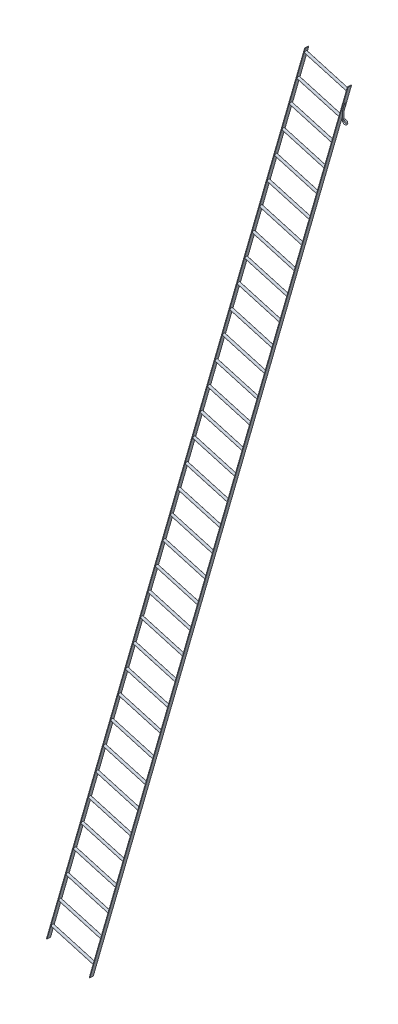
from build123d import *

# Parameters (mm, degrees)
SWEEP2_PROFILE_R                              = 6
CHAMFER1_SIZE                                 = 0.5
SKETCH1_W                                     = 40
SKETCH1_H                                     = 6
GB_T_704_1988HOT_ROLLED_FLAT_STEEL_40_6_DEPTH = 10400
SKETCH1_ON_SEGMENT_2_W                        = 40
SKETCH1_ON_SEGMENT_2_H                        = 6
GB_T_704_1988HOT_ROLLED_FLAT_STEEL_4_2_DEPTH  = 10400
SKETCH13_R                                    = 13.4
SKETCH13_R_2                                  = 10.4
GB_T_6728_2002ROUND_TUBE_26_8_X_3_2_DEPTH     = 494
SKETCH13_ON_SEGMENT_2_R                       = 13.4
SKETCH13_ON_SEGMENT_2_R_2                     = 10.4
GB_T_6728_2002ROUND_TUBE_26_8_X_3_2_2_DEPTH   = 494
PATTERN_LINEAR_1_COUNT                        = 34
PATTERN_LINEAR_1_PITCH                        = 300


with BuildPart() as part:
    # Sweep2: sweep along a path in feature 17 (ProfileFeature) (+16 more in 12 files) Sketch1
    with BuildLine(Plane.XY) as sweep2_path:
        Line((2.366140089, 179), (-19.767570176, 101.810579127))
        ThreePointArc((-19.767570176, 101.810579127), (-19.941608412, 100.991793598), (-20, 100.156754992))
        Line((-20, 100.156754992), (-20, 0))
        ThreePointArc((-20, 0), (14.142135624, -14.142135624), (0, 20))
        Line((0, 20), (-13.95, 20))
    # Sweep2 profile (on start of the path) → Sweep2 (sweep)
    with BuildSketch(Plane(origin=(2.366140089, 179, 0), x_dir=(-0.9612616959383187, 0.27563735581700005, 0), z_dir=(-0.27563735581700005, -0.9612616959383187, 0))):
        Circle(SWEEP2_PROFILE_R)
    sweep(path=sweep2_path.line)

    # Chamfer1
    chamfer1_edges = [part.edges().sort_by_distance(p)[0] for p in [
        (8.133710265, 177.346175865, 0),
    ]]
    chamfer(chamfer1_edges, length=CHAMFER1_SIZE)


with BuildPart() as body_2:
    # Sketch1 → Gb／t 704—1988Hot-rolled Flat Steel 40×6(1) (new body)
    with BuildSketch(Plane(origin=(-2816.280646199, -9629.021782916, -20), x_dir=(0, 0, 1), z_dir=(-0.27563735581699317, -0.9612616959383207, 0))):
        with Locations((20, 3)):
            Rectangle(SKETCH1_W, SKETCH1_H)
    extrude(amount=-GB_T_704_1988HOT_ROLLED_FLAT_STEEL_40_6_DEPTH)


with BuildPart() as body_3:
    # Sketch1 on segment 2 (carried to segment 2) → Gb_t 704_1988Hot-rolled Flat Steel 4 2 (new body)
    with BuildSketch(Plane(origin=(-424.515423496, 504.264708616, -20), x_dir=(0, 0, 1), z_dir=(-0.275637356, -0.961261696, 0))):
        with Locations((20, 3)):
            Rectangle(SKETCH1_ON_SEGMENT_2_W, SKETCH1_ON_SEGMENT_2_H)
    extrude(amount=GB_T_704_1988HOT_ROLLED_FLAT_STEEL_4_2_DEPTH)


with BuildPart() as body_4:
    # Sketch13 → Gb／t 6728—2002Round Tube 26.8 X 3(2) (new body)
    with BuildSketch(Plane(origin=(-3249.79832062, -9348.667674751, 0), x_dir=(0.2756373558170015, 0.9612616959383183, 0), z_dir=(0.9612616959383183, -0.2756373558170015, 0))):
        Circle(SKETCH13_R)
        Circle(SKETCH13_R_2, mode=Mode.SUBTRACT)
    extrude(amount=GB_T_6728_2002ROUND_TUBE_26_8_X_3_2_DEPTH)

    # Trim_Extend1 15
    split(bisect_by=Plane(origin=(-56.776544157, 16.280412056, 0), x_dir=(-0.275637356, -0.961261696, 0), z_dir=(-0.961261696, 0.275637356, 0)), keep=Keep.TOP)


with BuildPart() as body_5:
    # Sketch13 on segment 2 (carried to segment 2) → Gb_t 6728_2002Round Tube 26.8 X 3_2 2 (new body)
    with BuildSketch(Plane(origin=(-3167.107113875, -9060.28916597, 0), x_dir=(0.275637356, 0.961261696, 0), z_dir=(0.961261696, -0.275637356, 0))):
        Circle(SKETCH13_ON_SEGMENT_2_R)
        Circle(SKETCH13_ON_SEGMENT_2_R_2, mode=Mode.SUBTRACT)
    extrude(amount=GB_T_6728_2002ROUND_TUBE_26_8_X_3_2_2_DEPTH)

    # Trim_Extend1 15
    split(bisect_by=Plane(origin=(-56.776544157, 16.280412056, 0), x_dir=(-0.275637356, -0.961261696, 0), z_dir=(-0.961261696, 0.275637356, 0)), keep=Keep.TOP)


with BuildPart() as pattern_linear_1_1:
    # Pattern (Linear)1: pattern copy
    add(body_5.part.moved(Location(Vector(0.275637355817002, 0.9612616959383181, 0) * (1 * PATTERN_LINEAR_1_PITCH))))


with BuildPart() as pattern_linear_1_2:
    # Pattern (Linear)1: pattern copy
    add(body_5.part.moved(Location(Vector(0.275637355817002, 0.9612616959383181, 0) * (2 * PATTERN_LINEAR_1_PITCH))))


with BuildPart() as pattern_linear_1_3:
    # Pattern (Linear)1: pattern copy
    add(body_5.part.moved(Location(Vector(0.275637355817002, 0.9612616959383181, 0) * (3 * PATTERN_LINEAR_1_PITCH))))


with BuildPart() as pattern_linear_1_4:
    # Pattern (Linear)1: pattern copy
    add(body_5.part.moved(Location(Vector(0.275637355817002, 0.9612616959383181, 0) * (4 * PATTERN_LINEAR_1_PITCH))))


with BuildPart() as pattern_linear_1_5:
    # Pattern (Linear)1: pattern copy
    add(body_5.part.moved(Location(Vector(0.275637355817002, 0.9612616959383181, 0) * (5 * PATTERN_LINEAR_1_PITCH))))


with BuildPart() as pattern_linear_1_6:
    # Pattern (Linear)1: pattern copy
    add(body_5.part.moved(Location(Vector(0.275637355817002, 0.9612616959383181, 0) * (6 * PATTERN_LINEAR_1_PITCH))))


with BuildPart() as pattern_linear_1_7:
    # Pattern (Linear)1: pattern copy
    add(body_5.part.moved(Location(Vector(0.275637355817002, 0.9612616959383181, 0) * (7 * PATTERN_LINEAR_1_PITCH))))


with BuildPart() as pattern_linear_1_8:
    # Pattern (Linear)1: pattern copy
    add(body_5.part.moved(Location(Vector(0.275637355817002, 0.9612616959383181, 0) * (8 * PATTERN_LINEAR_1_PITCH))))


with BuildPart() as pattern_linear_1_9:
    # Pattern (Linear)1: pattern copy
    add(body_5.part.moved(Location(Vector(0.275637355817002, 0.9612616959383181, 0) * (9 * PATTERN_LINEAR_1_PITCH))))


with BuildPart() as pattern_linear_1_10:
    # Pattern (Linear)1: pattern copy
    add(body_5.part.moved(Location(Vector(0.275637355817002, 0.9612616959383181, 0) * (10 * PATTERN_LINEAR_1_PITCH))))


with BuildPart() as pattern_linear_1_11:
    # Pattern (Linear)1: pattern copy
    add(body_5.part.moved(Location(Vector(0.275637355817002, 0.9612616959383181, 0) * (11 * PATTERN_LINEAR_1_PITCH))))


with BuildPart() as pattern_linear_1_12:
    # Pattern (Linear)1: pattern copy
    add(body_5.part.moved(Location(Vector(0.275637355817002, 0.9612616959383181, 0) * (12 * PATTERN_LINEAR_1_PITCH))))


with BuildPart() as pattern_linear_1_13:
    # Pattern (Linear)1: pattern copy
    add(body_5.part.moved(Location(Vector(0.275637355817002, 0.9612616959383181, 0) * (13 * PATTERN_LINEAR_1_PITCH))))


with BuildPart() as pattern_linear_1_14:
    # Pattern (Linear)1: pattern copy
    add(body_5.part.moved(Location(Vector(0.275637355817002, 0.9612616959383181, 0) * (14 * PATTERN_LINEAR_1_PITCH))))


with BuildPart() as pattern_linear_1_15:
    # Pattern (Linear)1: pattern copy
    add(body_5.part.moved(Location(Vector(0.275637355817002, 0.9612616959383181, 0) * (15 * PATTERN_LINEAR_1_PITCH))))


with BuildPart() as pattern_linear_1_16:
    # Pattern (Linear)1: pattern copy
    add(body_5.part.moved(Location(Vector(0.275637355817002, 0.9612616959383181, 0) * (16 * PATTERN_LINEAR_1_PITCH))))


with BuildPart() as pattern_linear_1_17:
    # Pattern (Linear)1: pattern copy
    add(body_5.part.moved(Location(Vector(0.275637355817002, 0.9612616959383181, 0) * (17 * PATTERN_LINEAR_1_PITCH))))


with BuildPart() as pattern_linear_1_18:
    # Pattern (Linear)1: pattern copy
    add(body_5.part.moved(Location(Vector(0.275637355817002, 0.9612616959383181, 0) * (18 * PATTERN_LINEAR_1_PITCH))))


with BuildPart() as pattern_linear_1_19:
    # Pattern (Linear)1: pattern copy
    add(body_5.part.moved(Location(Vector(0.275637355817002, 0.9612616959383181, 0) * (19 * PATTERN_LINEAR_1_PITCH))))


with BuildPart() as pattern_linear_1_20:
    # Pattern (Linear)1: pattern copy
    add(body_5.part.moved(Location(Vector(0.275637355817002, 0.9612616959383181, 0) * (20 * PATTERN_LINEAR_1_PITCH))))


with BuildPart() as pattern_linear_1_21:
    # Pattern (Linear)1: pattern copy
    add(body_5.part.moved(Location(Vector(0.275637355817002, 0.9612616959383181, 0) * (21 * PATTERN_LINEAR_1_PITCH))))


with BuildPart() as pattern_linear_1_22:
    # Pattern (Linear)1: pattern copy
    add(body_5.part.moved(Location(Vector(0.275637355817002, 0.9612616959383181, 0) * (22 * PATTERN_LINEAR_1_PITCH))))


with BuildPart() as pattern_linear_1_23:
    # Pattern (Linear)1: pattern copy
    add(body_5.part.moved(Location(Vector(0.275637355817002, 0.9612616959383181, 0) * (23 * PATTERN_LINEAR_1_PITCH))))


with BuildPart() as pattern_linear_1_24:
    # Pattern (Linear)1: pattern copy
    add(body_5.part.moved(Location(Vector(0.275637355817002, 0.9612616959383181, 0) * (24 * PATTERN_LINEAR_1_PITCH))))


with BuildPart() as pattern_linear_1_25:
    # Pattern (Linear)1: pattern copy
    add(body_5.part.moved(Location(Vector(0.275637355817002, 0.9612616959383181, 0) * (25 * PATTERN_LINEAR_1_PITCH))))


with BuildPart() as pattern_linear_1_26:
    # Pattern (Linear)1: pattern copy
    add(body_5.part.moved(Location(Vector(0.275637355817002, 0.9612616959383181, 0) * (26 * PATTERN_LINEAR_1_PITCH))))


with BuildPart() as pattern_linear_1_27:
    # Pattern (Linear)1: pattern copy
    add(body_5.part.moved(Location(Vector(0.275637355817002, 0.9612616959383181, 0) * (27 * PATTERN_LINEAR_1_PITCH))))


with BuildPart() as pattern_linear_1_28:
    # Pattern (Linear)1: pattern copy
    add(body_5.part.moved(Location(Vector(0.275637355817002, 0.9612616959383181, 0) * (28 * PATTERN_LINEAR_1_PITCH))))


with BuildPart() as pattern_linear_1_29:
    # Pattern (Linear)1: pattern copy
    add(body_5.part.moved(Location(Vector(0.275637355817002, 0.9612616959383181, 0) * (29 * PATTERN_LINEAR_1_PITCH))))


with BuildPart() as pattern_linear_1_30:
    # Pattern (Linear)1: pattern copy
    add(body_5.part.moved(Location(Vector(0.275637355817002, 0.9612616959383181, 0) * (30 * PATTERN_LINEAR_1_PITCH))))


with BuildPart() as pattern_linear_1_31:
    # Pattern (Linear)1: pattern copy
    add(body_5.part.moved(Location(Vector(0.275637355817002, 0.9612616959383181, 0) * (31 * PATTERN_LINEAR_1_PITCH))))


with BuildPart() as pattern_linear_1_32:
    # Pattern (Linear)1: pattern copy
    add(body_5.part.moved(Location(Vector(0.275637355817002, 0.9612616959383181, 0) * (32 * PATTERN_LINEAR_1_PITCH))))


with BuildPart() as pattern_linear_1_33:
    # Pattern (Linear)1: pattern copy
    add(body_5.part.moved(Location(Vector(0.275637355817002, 0.9612616959383181, 0) * (33 * PATTERN_LINEAR_1_PITCH))))


solid = Compound([part.part, body_2.part, body_3.part, body_4.part, body_5.part, pattern_linear_1_1.part, pattern_linear_1_2.part, pattern_linear_1_3.part, pattern_linear_1_4.part, pattern_linear_1_5.part, pattern_linear_1_6.part, pattern_linear_1_7.part, pattern_linear_1_8.part, pattern_linear_1_9.part, pattern_linear_1_10.part, pattern_linear_1_11.part, pattern_linear_1_12.part, pattern_linear_1_13.part, pattern_linear_1_14.part, pattern_linear_1_15.part, pattern_linear_1_16.part, pattern_linear_1_17.part, pattern_linear_1_18.part, pattern_linear_1_19.part, pattern_linear_1_20.part, pattern_linear_1_21.part, pattern_linear_1_22.part, pattern_linear_1_23.part, pattern_linear_1_24.part, pattern_linear_1_25.part, pattern_linear_1_26.part, pattern_linear_1_27.part, pattern_linear_1_28.part, pattern_linear_1_29.part, pattern_linear_1_30.part, pattern_linear_1_31.part, pattern_linear_1_32.part, pattern_linear_1_33.part])
